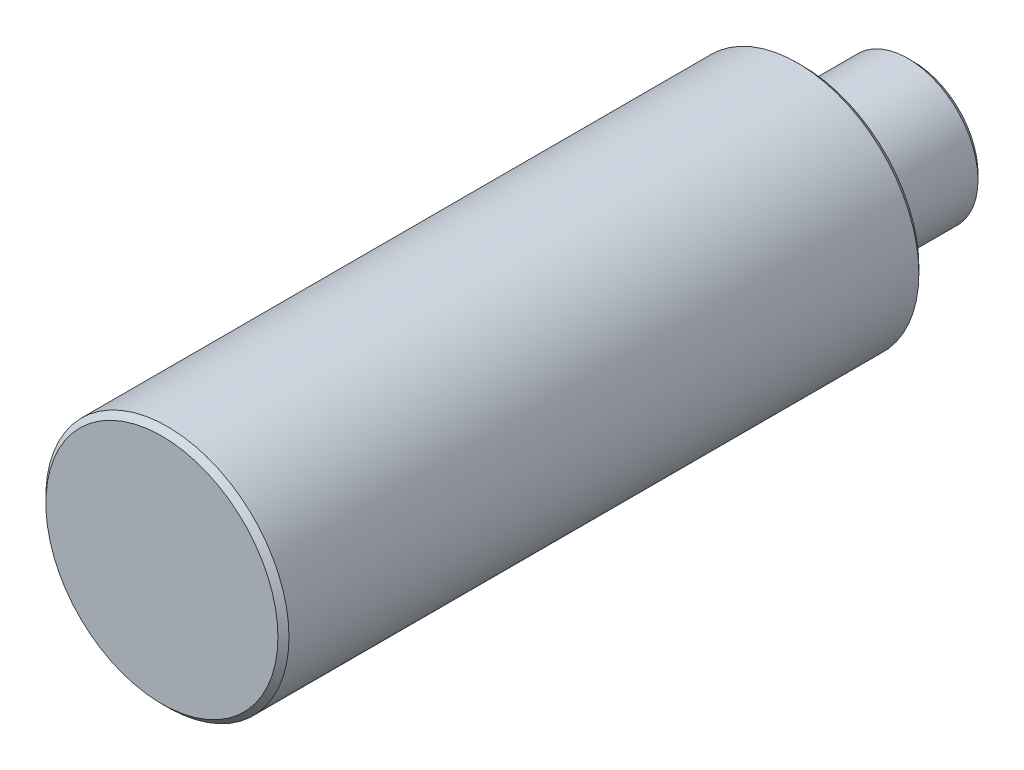
from build123d import *

# Parameters (mm, degrees)
SKETCH1_R           = 6.35
BOSS_EXTRUDE1_DEPTH = 10
SKETCH2_R           = 11
BOSS_EXTRUDE2_DEPTH = 58
CHAMFER1_SIZE       = 0.5


with BuildPart() as part:
    # Sketch1 → Boss-Extrude1 (new body)
    with BuildSketch(Plane.XY):
        Circle(SKETCH1_R)
    extrude(amount=BOSS_EXTRUDE1_DEPTH)

    # Sketch2 → Boss-Extrude2 (add)
    with BuildSketch(Plane.XY.offset(10)):
        Circle(SKETCH2_R)
    extrude(amount=BOSS_EXTRUDE2_DEPTH)

    # Chamfer1
    chamfer1_edges = [part.edges().sort_by_distance(p)[0] for p in [
        (-6.35, 0, 0),
        (-11, 0, 10),
        (-11, 0, 68),
    ]]
    chamfer(chamfer1_edges, length=CHAMFER1_SIZE)


solid = part.part
